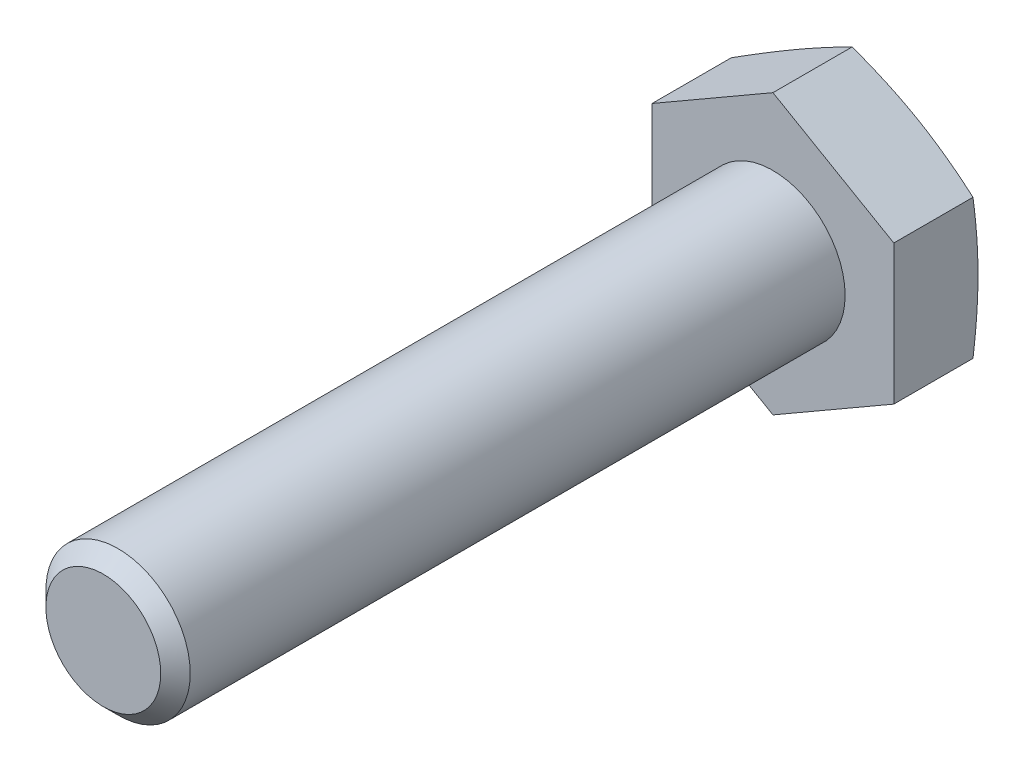
from build123d import *

# Parameters (mm, degrees)
SKETCH_2_R          = 11.6
CUT_EXTRUDE_1_DEPTH = 3.5


with BuildPart() as part:
    # 草图1 → 旋转1 (revolve)
    with BuildSketch(Plane(origin=(0, 0, 0), x_dir=(0, 0, -1), z_dir=(1, 0, 0)), mode=Mode.PRIVATE) as revolve_1_sk:
        Polygon((-9.333333333, 0), (-9.333333333, 2.3865), (-8.719833333, 3), (18.5, 3), (18.5, 5.8), (21.791789368, 5.8), (22, 5.022947342), (22, 0), align=None)
    revolve(revolve_1_sk.sketch.rotate(Axis((0, 0, -22), (0, 0, 1)), 270), axis=Axis((0, 0, -22), (0, 0, 1)))

    # 草图2 → 切除-拉伸1 (cut)
    with BuildSketch(Plane(origin=(0, 0, -22), x_dir=(-1, 0, 0), z_dir=(0, 0, -1))):
        Circle(SKETCH_2_R)
        Polygon((0, -5.8), (5.022947342, -2.9), (5.022947342, 2.9), (0, 5.8), (-5.022947342, 2.9), (-5.022947342, -2.9), align=None, mode=Mode.SUBTRACT)
    extrude(amount=-CUT_EXTRUDE_1_DEPTH, mode=Mode.SUBTRACT)


solid = part.part
